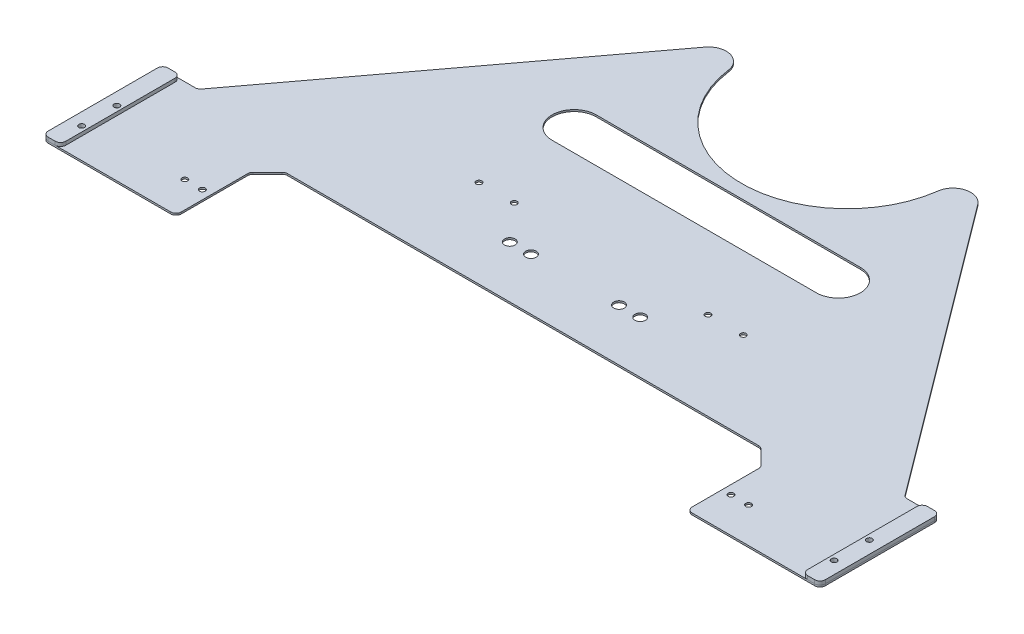
SolidWorks part; units mm, degrees
material "哈碳纤"
ref_plane "前视基准面" through (0, 0, 0) normal (0, 0, 1) x (1, 0, 0)
ref_plane "上视基准面" through (0, 0, 0) normal (0, 1, 0) x (1, 0, 0)
ref_plane "右视基准面" through (0, 0, 0) normal (1, 0, 0) x (0, 0, -1)
other "Configuration Table"
sketch "草图1" plane through (0, 0, 0) normal (0, 1, 0) x (1, 0, 0)
  line L0 (0, -303.695) -> (0, 14881.0565) construction
  line L1 (-135, 52) -> (135, 52)
  line L2 (145, 42) -> (145, 0)
  line L3 (-145, 42) -> (-145, 0)
  line L4 (145, 0) -> (220.55, 0)
  line L5 (-145, 0) -> (-220.55, 0)
  line L6 (220.55, 0) -> (220.55, 68)
  line L7 (-220.55, 0) -> (-220.55, 68)
  line L8 (220.55, 68) -> (200.55, 68)
  line L9 (-220.55, 68) -> (-200.55, 68)
  line L10 (200.55, 68) -> (77.3893, 232.6988)
  line L11 (-200.55, 68) -> (-77.3893, 232.6988)
  line L12 (135, 52) -> (145, 42)
  line L13 (-145, 42) -> (-135, 52)
  arc A0 (-59.4693, 228.0372) -> (59.4693, 228.0372) centre (0, 236) ccw
  arc A1 (-77.3893, 232.6988) -> (-59.4693, 228.0372) centre (-69.3808, 226.7101) cw
  arc A2 (77.3893, 232.6988) -> (59.4693, 228.0372) centre (69.3808, 226.7101) ccw
  circle A3 centre (213.55, 35) radius 1.6
  circle A4 centre (-213.55, 35) radius 1.6
  circle A5 centre (213.55, 15) radius 1.6
  circle A6 centre (-213.55, 15) radius 1.6
  point P4 (145, 52)
  point P5 (-145, 52)
  point P19 (-48.0508, 271.9321)
  point P22 (48.0508, 271.9321)
  dimension "D1" = 236
  dimension "D3" = 120
  dimension "D8" = 10
  dimension "D9" = 3.2
  dimension "D2" = 441.1
  dimension "D4" = 290
  dimension "D5" = 52
  dimension "D6" = 68
  dimension "D7" = 20
  dimension "D10" = 20
  dimension "D11" = 7
  dimension "D12" = 15
extrude "凸台-拉伸1" add sketch "草图1" along normal blind 1
sketch "草图2" plane through (0, 1, 0) normal (0, 1, 0) x (1, 0, 0)
  line L0 (0, 176) -> (0, 52) construction
  line L1 (-135, 52) -> (135, 52) construction
  line L2 (-75, 156) -> (75, 156) construction
  line L3 (-75, 168.5) -> (75, 168.5)
  line L4 (-75, 143.5) -> (75, 143.5)
  line L5 (-55, 102) -> (55, 102) construction
  line L6 (-220.55, 0) -> (-145, 0) construction
  arc A0 (-59.4693, 228.0372) -> (59.4693, 228.0372) centre (0, 236) ccw construction
  arc A1 (-75, 168.5) -> (-75, 143.5) centre (-75, 156) ccw
  arc A2 (75, 143.5) -> (75, 168.5) centre (75, 156) ccw
  circle A3 centre (-55, 102) radius 1.6
  circle A4 centre (-75, 102) radius 1.6
  circle A5 centre (75, 102) radius 1.6
  circle A6 centre (55, 102) radius 1.6
  circle A7 centre (-25, 81.5) radius 3
  circle A8 centre (-37, 81.5) radius 3
  circle A9 centre (37, 81.5) radius 3
  circle A10 centre (25, 81.5) radius 3
  circle A11 centre (-160, 20) radius 1.6
  circle A12 centre (-150, 20) radius 1.6
  circle A13 centre (150, 20) radius 1.6
  circle A14 centre (160, 20) radius 1.6
  point P9 (0, 156)
  point P17 (0, 102)
  dimension "D6" = 3.2
  dimension "D7" = 20
  dimension "D8" = 20.5
  dimension "D10" = 6
  dimension "D12" = 10
  dimension "D13" = 3.2
  dimension "D1" = 25
  dimension "D2" = 150
  dimension "D3" = 104
  dimension "D4" = 110
  dimension "D5" = 50
  dimension "D9" = 30
  dimension "D11" = 12
  dimension "D14" = 20
  dimension "D15" = 300
extrude "切除-拉伸1" cut sketch "草图2" against normal blind 10
fillet "圆角1" radius 3 12 edges at (145, 0.5, -42) (135, 0.5, -52) (-135, 0.5, -52) (-145, 0.5, -42) (-145, 0.5, 0) (-220.55, 0.5, 0) (-220.55, 0.5, -68) (-200.55, 0.5, -68) (200.55, 0.5, -68) (220.55, 0.5, -68) (220.55, 0.5, 0) (145, 0.5, 0)
sketch "草图3" plane through (0, 1, 0) normal (0, 1, 0) x (1, 0, 0)
  line L0 (148, 0) -> (217.55, 0) construction
  line L1 (213.55, 0) -> (217.55, 0)
  line L2 (210.55, 3) -> (210.55, 65)
  line L3 (213.55, 68) -> (217.55, 68)
  line L4 (220.55, 3) -> (220.55, 65)
  line L5 (220.55, 3) -> (220.55, 65) construction
  line L6 (217.55, 68) -> (202.0527, 68) construction
  arc A0 (217.55, 0) -> (220.55, 3) centre (217.55, 3) ccw
  arc A1 (210.55, 65) -> (213.55, 68) centre (213.55, 65) cw
  arc A2 (217.55, 68) -> (220.55, 65) centre (217.55, 65) cw
  arc A3 (213.55, 0) -> (210.55, 3) centre (213.55, 3) cw
  circle A4 centre (213.55, 15) radius 1.6 construction
  circle A5 centre (213.55, 35) radius 1.6 construction
  circle A6 centre (213.55, 15) radius 1.6
  circle A7 centre (213.55, 35) radius 1.6
  point P18 (210.55, 0)
  dimension "D2" = 3
  dimension "D1" = 10
extrude "凸台-拉伸2" add sketch "草图3" along normal blind 2 separate body
mirror "镜向1" about plane through (0, 0, 0) normal (1, 0, 0) of bodies 108
